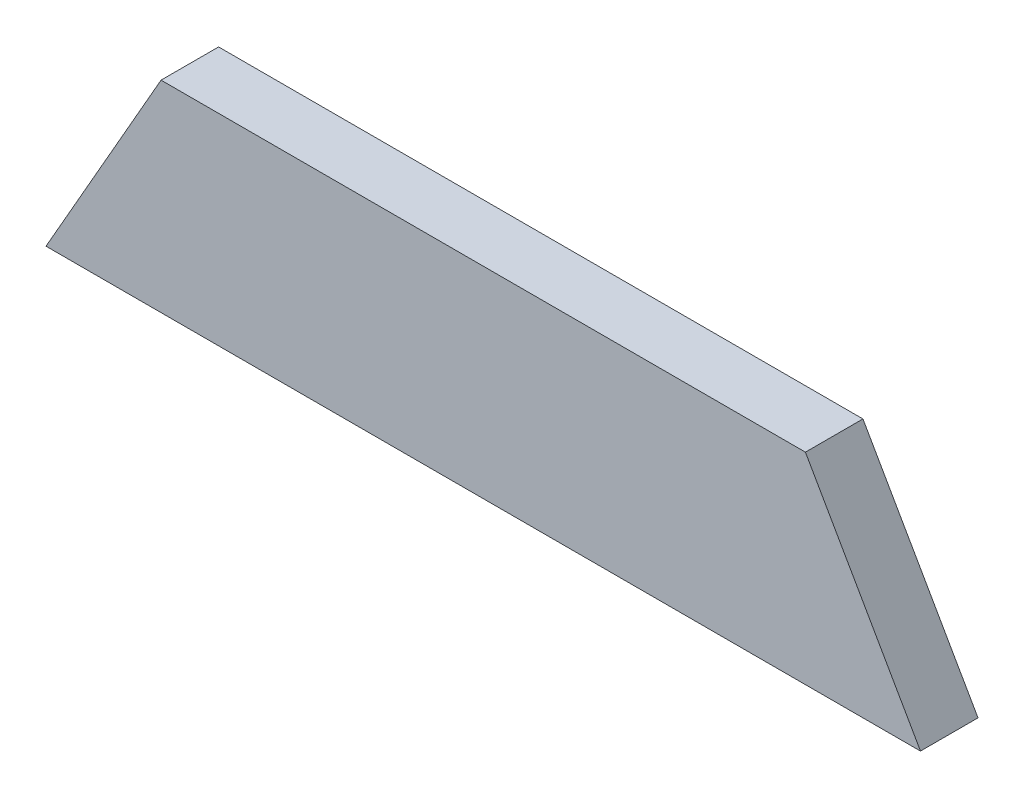
from build123d import *

# Parameters (mm, degrees)
BOSS_EXTRUDE1_DEPTH = 10


with BuildPart() as part:
    # Sketch1 → Boss-Extrude1 (new body)
    with BuildSketch(Plane.XY):
        Polygon((0, 0), (152, 0), (132, 35), (20, 35), align=None)
    extrude(amount=BOSS_EXTRUDE1_DEPTH)


solid = part.part
